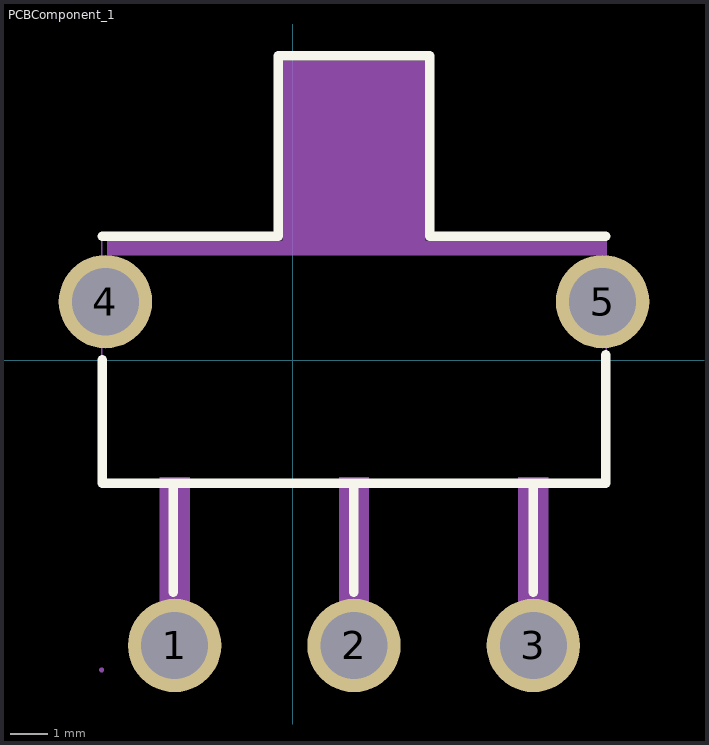
[diagram p0: the footprint, top view; thin cyan lines are the x and y axes]
# Altium footprint library MISC82341-18.PcbLib: 1 footprints
Each footprint in its own frame and in the unit in brackets; x right, y up, seen from the top. Pads: shape width x height; smd on the part's side, far side on the other; paste and mask are expansions set on the pad; w line width, h text height; cw(c..) or ccw(c..) is an arc to the next point about the centre after c.

## PCBComponent_1 [mm]
pads (5):
  round 2.5 hole 1.8: 1(-3.159,-7.63) 2(1.641,-7.63) 3(6.441,-7.63) 4(-5.009,1.57) 5(8.291,1.57)
Top Overlay:
  lines w0.254: -5.09,0.018 -5.09,-3.284 8.372,-3.284 8.372,0.145 ; -5.09,3.32 -0.391,3.32 -0.391,8.146 3.673,8.146 3.673,3.32 8.372,3.32 ; -3.194,-6.205 -3.194,-3.284 ; 1.632,-6.205 1.632,-3.284 ; 6.432,-6.205 6.432,-3.284
Mechanical 6:
  region: -4.963,3.193 8.372,3.193 8.372,2.812 -4.963,2.812
  region: -0.264,8.019 -0.264,3.193 3.546,3.193 3.546,8.019
Mechanical 15:
  region: -3.559,-3.13 -2.759,-3.13 -2.759,-8.28 -3.559,-8.28
  region: 1.241,-3.13 2.041,-3.13 2.041,-8.28 1.241,-8.28
  region: 6.041,-3.13 6.841,-3.13 6.841,-8.28 6.041,-8.28
  region: 1.241,-6.98 2.041,-6.98 2.041,-8.28 1.241,-8.28
  region: 8.191,2.195 8.391,2.195 8.391,0.945 8.191,0.945
  region: -5.109,2.195 -4.909,2.195 -4.909,0.945 -5.109,0.945
  region: 6.041,-6.98 6.841,-6.98 6.841,-8.28 6.041,-8.28
  region: -3.559,-6.98 -2.759,-6.98 -2.759,-8.28 -3.559,-8.28
  region: -5.049,-8.28 -5.049,-8.255 -5.084,-8.22 -5.134,-8.22 -5.169,-8.255 -5.169,-8.28 -5.169,-8.305 -5.134,-8.34 -5.084,-8.34 -5.049,-8.305 -5.049,-8.28
  lines w0.051: -5.109,-3.332 8.391,-3.332 8.391,3.268 3.741,3.27 3.741,8.096 -0.459,8.096 -0.459,3.27 -5.109,3.268 -5.109,-3.332